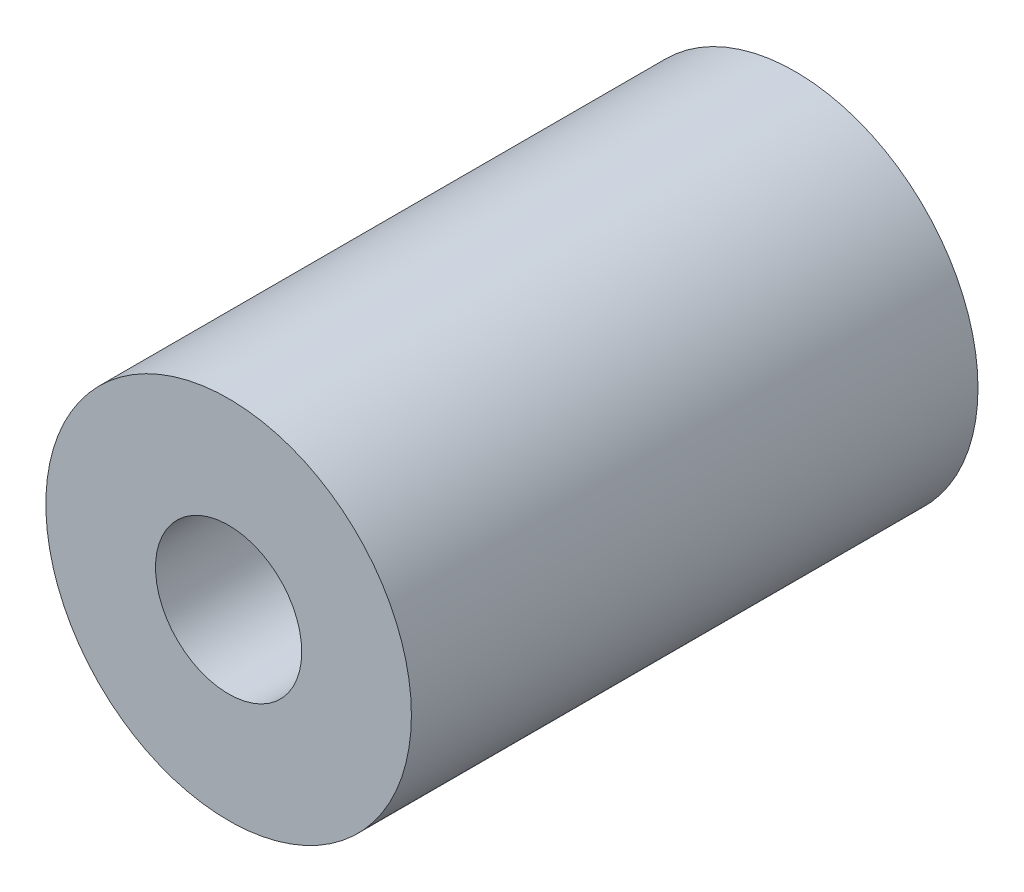
from build123d import *

# Parameters (mm, degrees)
SKETCH_1_R      = 5
SKETCH_1_R_2    = 2
EXTRUDE_1_DEPTH = 15.5


with BuildPart() as part:
    # 草图1 → 凸台-拉伸1 (new body)
    with BuildSketch(Plane.XY):
        Circle(SKETCH_1_R)
        Circle(SKETCH_1_R_2, mode=Mode.SUBTRACT)
    extrude(amount=EXTRUDE_1_DEPTH)


solid = part.part
